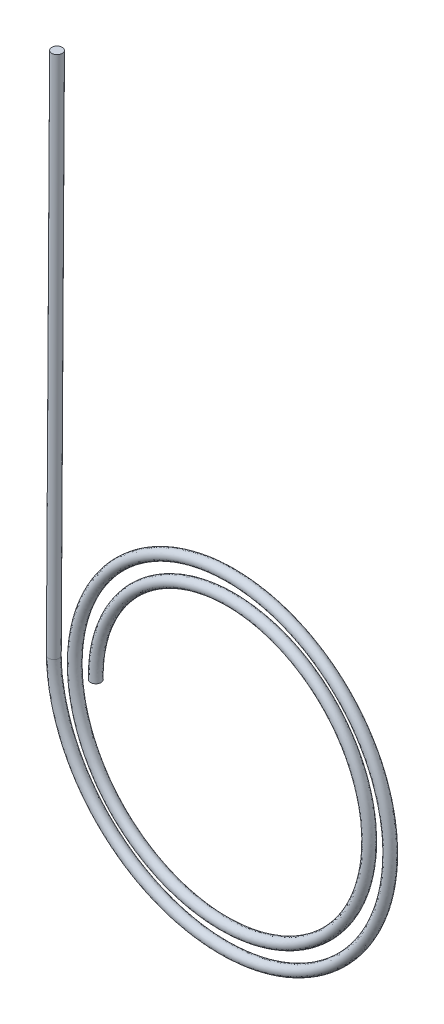
from build123d import *

# Parameters (mm, degrees)
SKETCH2_R           = 0.5
SKETCH3_R           = 0.5
BOSS_EXTRUDE1_DEPTH = 50


with BuildPart() as part:
    # Sweep1: sweep along a curve in space
    with BuildLine() as sweep1_path:
        add(Edge.make_bspline(
            [(-12.5, 0, 0), (-12.541666667, 1.636246174, 0), (-12.257910062, 3.288621897, 0), (-11.070048133, 6.37413477, 0), (-10.166289458, 7.806007897, 0), (-7.864933462, 10.225215023, 0), (-6.468149229, 11.21150477, 0), (-3.385949154, 12.578393193, 0), (-1.701696021, 12.958333333, 0), (1.701696021, 13.041666667, 0), (3.419495839, 12.744896401, 0), (6.62594426, 11.506941328, 0), (8.113281257, 10.566122879, 0), (10.625048444, 8.172206822, 0), (11.648397964, 6.719958719, 0), (13.065379531, 3.516823096, 0), (13.458333333, 1.767145868, 0), (13.541666667, -1.767145868, 0), (13.231882739, -3.550369781, 0), (11.943834522, -6.877753751, 0), (10.9659563, -8.420554617, 0), (8.479480182, -11.024881866, 0), (6.97176821, -12.085291158, 0), (3.647697039, -13.552365869, 0), (1.832595715, -13.958333333, 0), (-1.832595715, -14.041666667, 0), (-3.681243724, -13.718869077, 0), (-7.129563241, -12.380727716, 0), (-8.727827977, -11.365789722, 0), (-11.424715287, -8.786753542, 0), (-12.522184352, -7.2235777, 0), (-14.039352208, -3.778570981, 0), (-14.458333333, -1.898045562, 0), (-14.541666667, 1.898045562, 0), (-14.205855416, 3.812117666, 0), (-12.81762091, 7.381372731, 0), (-11.765623143, 9.035101337, 0), (-9.094026902, 11.824548708, 0), (-7.47538719, 12.959077546, 0), (-3.909444923, 14.526338546, 0), (-1.963495408, 14.958333333, 0), (1.963495408, 15.041666667, 0), (3.942991608, 14.692841754, 0), (7.633182221, 13.254514104, 0), (9.342374697, 12.165456564, 0), (12.224382129, 9.401300262, 0), (13.39597074, 7.72719668, 0), (15.013324884, 4.040318865, 0), (15.458333333, 2.028945255, 0), (15.541666667, -2.028945255, 0), (15.179828092, -4.07386555, 0), (13.691407299, -7.884991711, 0), (12.565289985, -9.649648057, 0), (9.708573622, -12.62421555, 0), (7.97900617, -13.832863935, 0), (4.171192807, -15.500311223, 0), (2.094395102, -15.958333333, 0), (-2.094395102, -16.041666667, 0), (-4.204739492, -15.666814431, 0), (-7.153785774, -14.512928977, 0), (-8.100802158, -14.030701726, 0), (-9.885784136, -12.888126973, 0), (-10.723703306, -12.2278043, 0), (-12.257267083, -10.753166088, 0), (-12.952870859, -9.9388841, 0), (-14.173825243, -8.186594752, 0), (-14.699142237, -7.248628433, 0), (-15.557912453, -5.284253977, 0), (-15.891340636, -4.257892838, 0), (-16.351975457, -2.155701498, 0), (-16.479166667, -1.079922475, 0), (-16.5, 0, 0)],
            knots=[0, 0, 0, 0, 0.03125, 0.03125, 0.0625, 0.0625, 0.09375, 0.09375, 0.125, 0.125, 0.15625, 0.15625, 0.1875, 0.1875, 0.21875, 0.21875, 0.25, 0.25, 0.28125, 0.28125, 0.3125, 0.3125, 0.34375, 0.34375, 0.375, 0.375, 0.40625, 0.40625, 0.4375, 0.4375, 0.46875, 0.46875, 0.5, 0.5, 0.53125, 0.53125, 0.5625, 0.5625, 0.59375, 0.59375, 0.625, 0.625, 0.65625, 0.65625, 0.6875, 0.6875, 0.71875, 0.71875, 0.75, 0.75, 0.78125, 0.78125, 0.8125, 0.8125, 0.84375, 0.84375, 0.875, 0.875, 0.90625, 0.90625, 0.921875, 0.921875, 0.9375, 0.9375, 0.953125, 0.953125, 0.96875, 0.96875, 0.984375, 0.984375, 1, 1, 1, 1], degree=3))
    # Sketch2 → Sweep1 (sweep)
    with BuildSketch(Plane(origin=(0, 0, 0), x_dir=(1, 0, 0), z_dir=(0, 1, 0))):
        with Locations((-12.5003961, 0)):
            Circle(SKETCH2_R)
    sweep(path=sweep1_path.line, is_frenet=True)

    # Sketch3 → Boss-Extrude1 (add)
    with BuildSketch(Plane(origin=(-0.000628109, -0.101802051, 0), x_dir=(0.9999809666609517, -0.006169790582240785, 0), z_dir=(0.006169790582240785, 0.9999809666609517, 0))):
        with Locations(Location((-16.500082042, 0, 0), (0, 0, 270))):
            Circle(SKETCH3_R)
    extrude(amount=BOSS_EXTRUDE1_DEPTH)


solid = part.part
